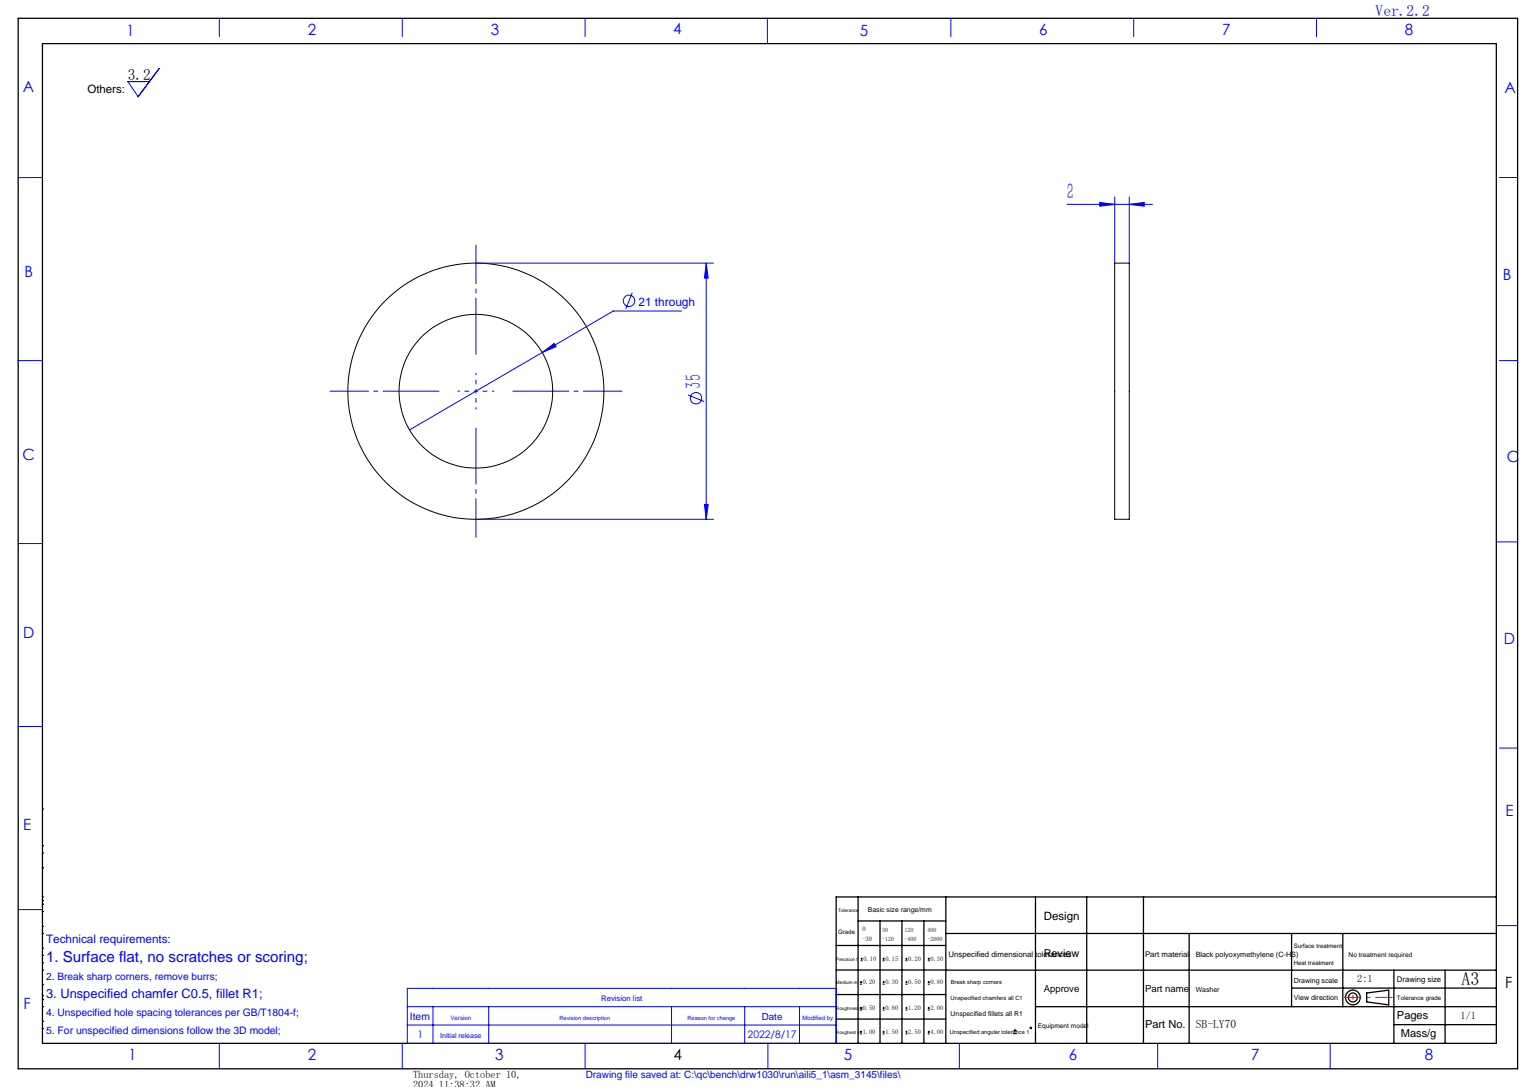
from build123d import *

# Parameters (mm, degrees)
SKETCH_1_R      = 17.5
SKETCH_1_R_2    = 10.5
EXTRUDE_1_DEPTH = 2


with BuildPart() as part:
    # 草图1 → 凸台-拉伸1 (new body)
    with BuildSketch(Plane.XY):
        Circle(SKETCH_1_R)
        Circle(SKETCH_1_R_2, mode=Mode.SUBTRACT)
    extrude(amount=EXTRUDE_1_DEPTH)


solid = part.part
